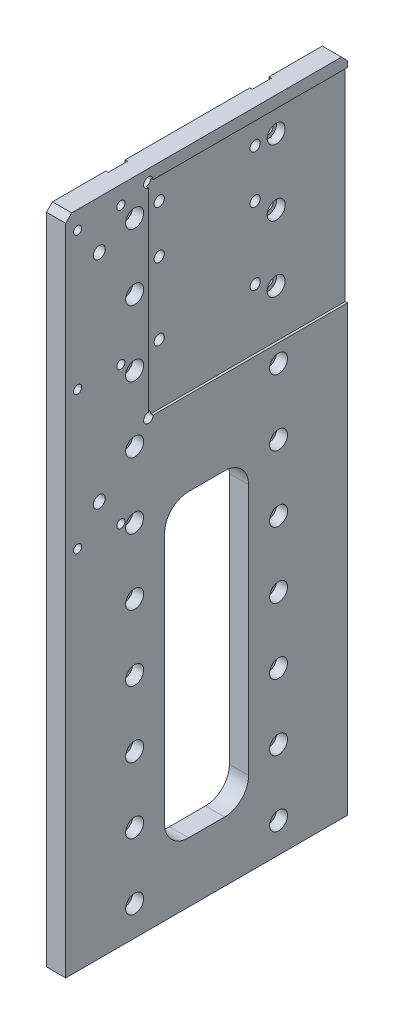
from build123d import *

# Parameters (mm, degrees)
SKETCH_1_W               = 16
SKETCH_1_H               = 550
EXTRUDE_1_DEPTH          = 235
SKETCH_4_W               = 16
SKETCH_4_H               = 550
CUT_EXTRUDE_3_DEPTH      = 2
SKETCH_5_W               = 166
SKETCH_5_H               = 170
CUT_EXTRUDE_4_DEPTH      = 2
HOLE_WIZARD_M10_1_D      = 8.5
HOLE_WIZARD_M10_1_DEPTH  = 27.5
HOLE_WIZARD_M10_1_TIP    = 2.553657631
HOLE_WIZARD_M8_1_D       = 6.8
HOLE_WIZARD_M8_1_DEPTH   = 22.25
HOLE_WIZARD_M8_1_TIP     = 2.042926105
SKETCH_15_W              = 70
SKETCH_15_H              = 250
CUT_EXTRUDE_5_DEPTH      = 16
FILLET_1_R               = 20
CHAMFER_1_SIZE           = 5
HOLE_WIZARD_1_AT_2_COUNT = 2
HOLE_WIZARD_1_AT_2_PITCH = 120
PATTERN_LINEAR_1_COUNT   = 10
PATTERN_LINEAR_1_PITCH   = 55
HOLE_WIZARD_M8_2_D       = 6.8
HOLE_WIZARD_M8_2_DEPTH   = 22.25
HOLE_WIZARD_M8_2_TIP     = 2.042926105
SKETCH_20_R              = 4
CUT_EXTRUDE_6_DEPTH      = 363.085625232
MM_1_D                   = 10
MM_1_DEPTH               = 10
MM_1_TIP                 = 3.004303095


with BuildPart() as part:
    # 草图1 → 凸台-拉伸1 (new body)
    with BuildSketch(Plane.XY):
        Rectangle(SKETCH_1_W, SKETCH_1_H)
    extrude(amount=EXTRUDE_1_DEPTH)

    # 草图4 → 切除-拉伸3 (cut)
    with BuildSketch(Plane.ZY.offset(8)):
        with Locations((57.5, 0)):
            Rectangle(SKETCH_4_W, SKETCH_4_H)
        with Locations((177.5, 0)):
            Rectangle(SKETCH_4_W, SKETCH_4_H)
    extrude(amount=-CUT_EXTRUDE_3_DEPTH, mode=Mode.SUBTRACT)

    # 草图5 → 切除-拉伸4 (cut)
    with BuildSketch(Plane(origin=(8, 0, 0), x_dir=(0, 0, -1), z_dir=(1, 0, 0))):
        with Locations((-83, 180)):
            Rectangle(SKETCH_5_W, SKETCH_5_H)
    extrude(amount=-CUT_EXTRUDE_4_DEPTH, mode=Mode.SUBTRACT)

    # M10 螺纹孔1
    with Locations(Plane(origin=(6, 0, 0), x_dir=(0, 0, -1), z_dir=(1, 0, 0))):
        with Locations((-155, 245), (-75, 145), (-155, 145), (-75, 245), (-75, 205), (-155, 205)):
            Hole(HOLE_WIZARD_M10_1_D / 2, depth=HOLE_WIZARD_M10_1_DEPTH)
            with Locations((0, 0, -(HOLE_WIZARD_M10_1_DEPTH + HOLE_WIZARD_M10_1_TIP / 2))):  # 118° drill point
                Cone(0, HOLE_WIZARD_M10_1_D / 2, HOLE_WIZARD_M10_1_TIP, mode=Mode.SUBTRACT)

    # M8 螺纹孔1
    with Locations(Plane(origin=(0, -275, 0), x_dir=(-1, 0, 0), z_dir=(0, -1, 0))):
        with Locations((0, -207.5), (0, -72.5), (0, -27.5), (0, -117.5), (0, -162.5)):
            Hole(HOLE_WIZARD_M8_1_D / 2, depth=HOLE_WIZARD_M8_1_DEPTH)
            with Locations((0, 0, -(HOLE_WIZARD_M8_1_DEPTH + HOLE_WIZARD_M8_1_TIP / 2))):  # 118° drill point
                Cone(0, HOLE_WIZARD_M8_1_D / 2, HOLE_WIZARD_M8_1_TIP, mode=Mode.SUBTRACT)

    # 草图15 → 切除-拉伸5 (cut)
    with BuildSketch(Plane.ZY.offset(8)):
        with Locations((117.5, -100)):
            Rectangle(SKETCH_15_W, SKETCH_15_H)
    extrude(amount=-CUT_EXTRUDE_5_DEPTH, mode=Mode.SUBTRACT)

    # 圆角1
    fillet_1_edges = [part.edges().sort_by_distance(p)[0] for p in [
        (0, 25, 152.5),
        (0, -225, 152.5),
        (0, -225, 82.5),
        (0, 25, 82.5),
    ]]
    fillet(fillet_1_edges, radius=FILLET_1_R)

    # 倒角1
    chamfer_1_edges = [part.edges().sort_by_distance(p)[0] for p in [
        (0, 275, 0),
        (0, 275, 235),
    ]]
    chamfer(chamfer_1_edges, length=CHAMFER_1_SIZE)

    # 草图17 → 打孔尺寸(%根据)内六角圆柱头螺钉的类型1 (revolve, cut)
    with BuildSketch(Plane(origin=(8, -250, 57.5), x_dir=(0, 0, -1), z_dir=(0, 1, 0))):
        Polygon((0, 0), (0, 30.203872786), (4.5, 27.5), (4.5, 9), (7.5, 9), (7.5, 0), align=None)
    hole_wizard_1 = revolve(axis=Axis((14.35, -250, 57.5), (-1, 0, 0)), mode=Mode.SUBTRACT)

    # 打孔尺寸(%根据)内六角圆柱头螺钉的类型1 at 2: 打孔尺寸(%根据)内六角圆柱头螺钉的类型1 ×2
    with Locations(*[(0, 0, i * HOLE_WIZARD_1_AT_2_PITCH) for i in range(1, HOLE_WIZARD_1_AT_2_COUNT)]):
        add(hole_wizard_1, mode=Mode.SUBTRACT)

    # 阵列(线性)1: 打孔尺寸(%根据)内六角圆柱头螺钉的类型1 ×10
    with Locations(*[(0, i * PATTERN_LINEAR_1_PITCH, 0) for i in range(1, PATTERN_LINEAR_1_COUNT)]):
        add(hole_wizard_1, mode=Mode.SUBTRACT)

    # 阵列(线性)1 copy 1 sketch → 阵列(线性)1 copy 1 (revolve, cut)
    with BuildSketch(Plane(origin=(8, -195, 177.5), x_dir=(0, 0, -1), z_dir=(0, 1, 0))):
        Polygon((0, 0), (0, 30.203872786), (4.5, 27.5), (4.5, 9), (7.5, 9), (7.5, 0), align=None)
    revolve(axis=Axis((14.35, -195, 177.5), (-1, 0, 0)), mode=Mode.SUBTRACT)

    # 阵列(线性)1 copy 2 sketch → 阵列(线性)1 copy 2 (revolve, cut)
    with BuildSketch(Plane(origin=(8, -140, 177.5), x_dir=(0, 0, -1), z_dir=(0, 1, 0))):
        Polygon((0, 0), (0, 30.203872786), (4.5, 27.5), (4.5, 9), (7.5, 9), (7.5, 0), align=None)
    revolve(axis=Axis((14.35, -140, 177.5), (-1, 0, 0)), mode=Mode.SUBTRACT)

    # 阵列(线性)1 copy 3 sketch → 阵列(线性)1 copy 3 (revolve, cut)
    with BuildSketch(Plane(origin=(8, -85, 177.5), x_dir=(0, 0, -1), z_dir=(0, 1, 0))):
        Polygon((0, 0), (0, 30.203872786), (4.5, 27.5), (4.5, 9), (7.5, 9), (7.5, 0), align=None)
    revolve(axis=Axis((14.35, -85, 177.5), (-1, 0, 0)), mode=Mode.SUBTRACT)

    # 阵列(线性)1 copy 4 sketch → 阵列(线性)1 copy 4 (revolve, cut)
    with BuildSketch(Plane(origin=(8, -30, 177.5), x_dir=(0, 0, -1), z_dir=(0, 1, 0))):
        Polygon((0, 0), (0, 30.203872786), (4.5, 27.5), (4.5, 9), (7.5, 9), (7.5, 0), align=None)
    revolve(axis=Axis((14.35, -30, 177.5), (-1, 0, 0)), mode=Mode.SUBTRACT)

    # 阵列(线性)1 copy 5 sketch → 阵列(线性)1 copy 5 (revolve, cut)
    with BuildSketch(Plane(origin=(8, 25, 177.5), x_dir=(0, 0, -1), z_dir=(0, 1, 0))):
        Polygon((0, 0), (0, 30.203872786), (4.5, 27.5), (4.5, 9), (7.5, 9), (7.5, 0), align=None)
    revolve(axis=Axis((14.35, 25, 177.5), (-1, 0, 0)), mode=Mode.SUBTRACT)

    # 阵列(线性)1 copy 6 sketch → 阵列(线性)1 copy 6 (revolve, cut)
    with BuildSketch(Plane(origin=(8, 80, 177.5), x_dir=(0, 0, -1), z_dir=(0, 1, 0))):
        Polygon((0, 0), (0, 30.203872786), (4.5, 27.5), (4.5, 9), (7.5, 9), (7.5, 0), align=None)
    revolve(axis=Axis((14.35, 80, 177.5), (-1, 0, 0)), mode=Mode.SUBTRACT)

    # 阵列(线性)1 copy 7 sketch → 阵列(线性)1 copy 7 (revolve, cut)
    with BuildSketch(Plane(origin=(8, 135, 177.5), x_dir=(0, 0, -1), z_dir=(0, 1, 0))):
        Polygon((0, 0), (0, 30.203872786), (4.5, 27.5), (4.5, 9), (7.5, 9), (7.5, 0), align=None)
    revolve(axis=Axis((14.35, 135, 177.5), (-1, 0, 0)), mode=Mode.SUBTRACT)

    # 阵列(线性)1 copy 8 sketch → 阵列(线性)1 copy 8 (revolve, cut)
    with BuildSketch(Plane(origin=(8, 190, 177.5), x_dir=(0, 0, -1), z_dir=(0, 1, 0))):
        Polygon((0, 0), (0, 30.203872786), (4.5, 27.5), (4.5, 9), (7.5, 9), (7.5, 0), align=None)
    revolve(axis=Axis((14.35, 190, 177.5), (-1, 0, 0)), mode=Mode.SUBTRACT)

    # 阵列(线性)1 copy 9 sketch → 阵列(线性)1 copy 9 (revolve, cut)
    with BuildSketch(Plane(origin=(8, 245, 177.5), x_dir=(0, 0, -1), z_dir=(0, 1, 0))):
        Polygon((0, 0), (0, 30.203872786), (4.5, 27.5), (4.5, 9), (7.5, 9), (7.5, 0), align=None)
    revolve(axis=Axis((14.35, 245, 177.5), (-1, 0, 0)), mode=Mode.SUBTRACT)

    # M8 螺纹孔2
    with Locations(Plane(origin=(8, 0, 0), x_dir=(0, 0, -1), z_dir=(1, 0, 0))):
        with Locations((-225, 30), (-189, 145), (-225, 145), (-189, 260), (-225, 260), (-189, 30)):
            Hole(HOLE_WIZARD_M8_2_D / 2, depth=HOLE_WIZARD_M8_2_DEPTH)
            with Locations((0, 0, -(HOLE_WIZARD_M8_2_DEPTH + HOLE_WIZARD_M8_2_TIP / 2))):  # 118° drill point
                Cone(0, HOLE_WIZARD_M8_2_D / 2, HOLE_WIZARD_M8_2_TIP, mode=Mode.SUBTRACT)

    # 草图20 → 切除-拉伸6 (cut, through all)
    with BuildSketch(Plane(origin=(8, 0, 0), x_dir=(0, 0, -1), z_dir=(1, 0, 0))):
        with Locations((-166, 95)):
            Circle(SKETCH_20_R)
        with Locations((-166, 265)):
            Circle(SKETCH_20_R)
    extrude(amount=-CUT_EXTRUDE_6_DEPTH, mode=Mode.SUBTRACT)

    # 大小mm 暗销孔1
    with Locations(Plane(origin=(8, 0, 0), x_dir=(0, 0, -1), z_dir=(1, 0, 0))):
        with Locations((-207, 235), (-207, 55)):
            Hole(MM_1_D / 2, depth=MM_1_DEPTH)
            with Locations((0, 0, -(MM_1_DEPTH + MM_1_TIP / 2))):  # 118° drill point
                Cone(0, MM_1_D / 2, MM_1_TIP, mode=Mode.SUBTRACT)


solid = part.part
